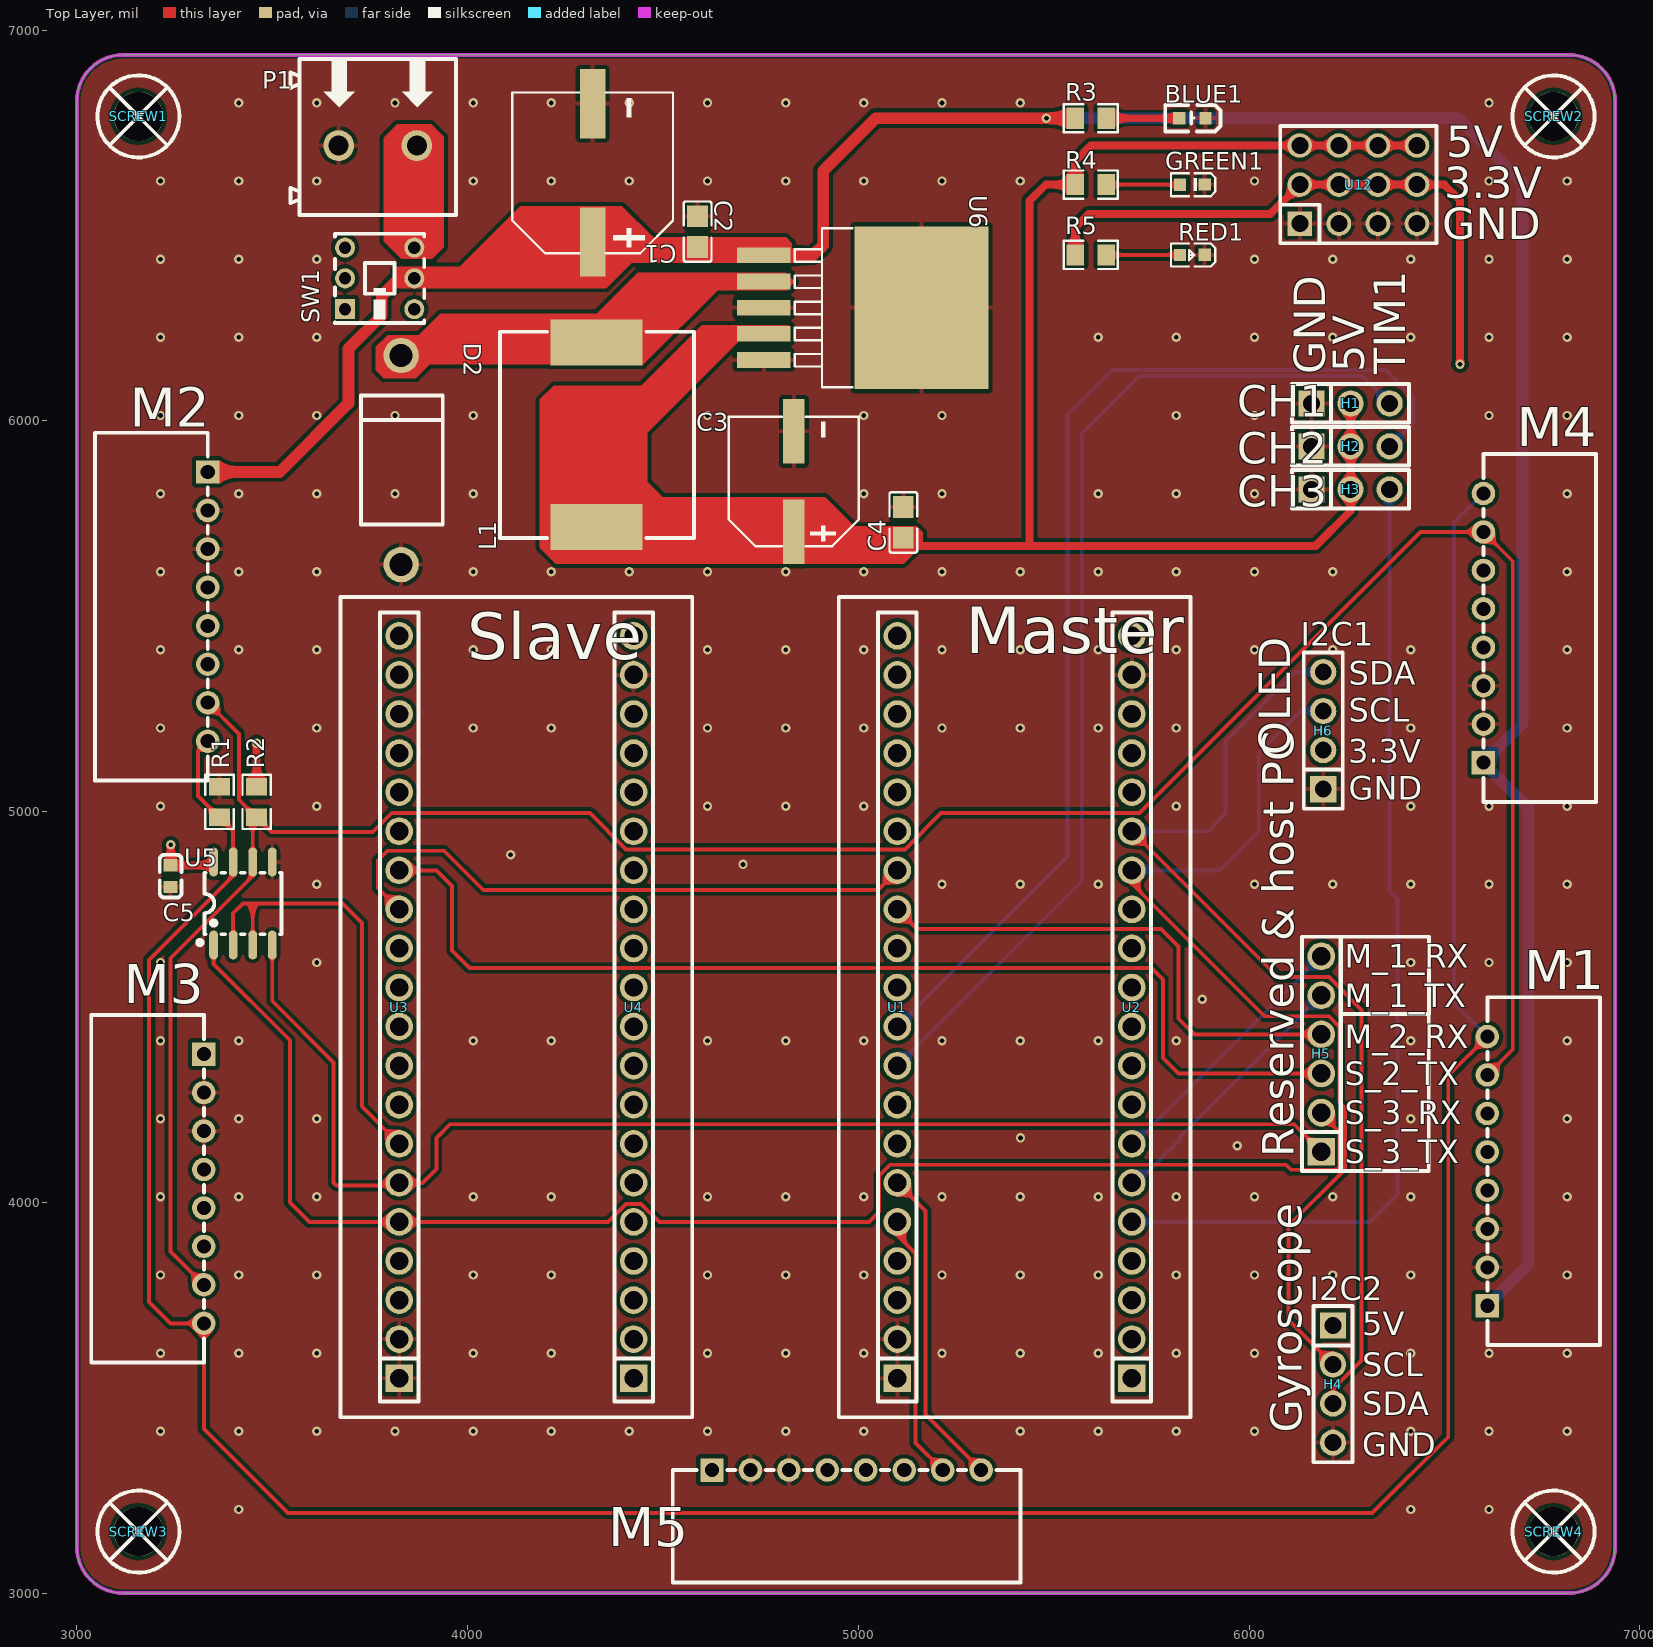
[diagram p0: Top Layer view]
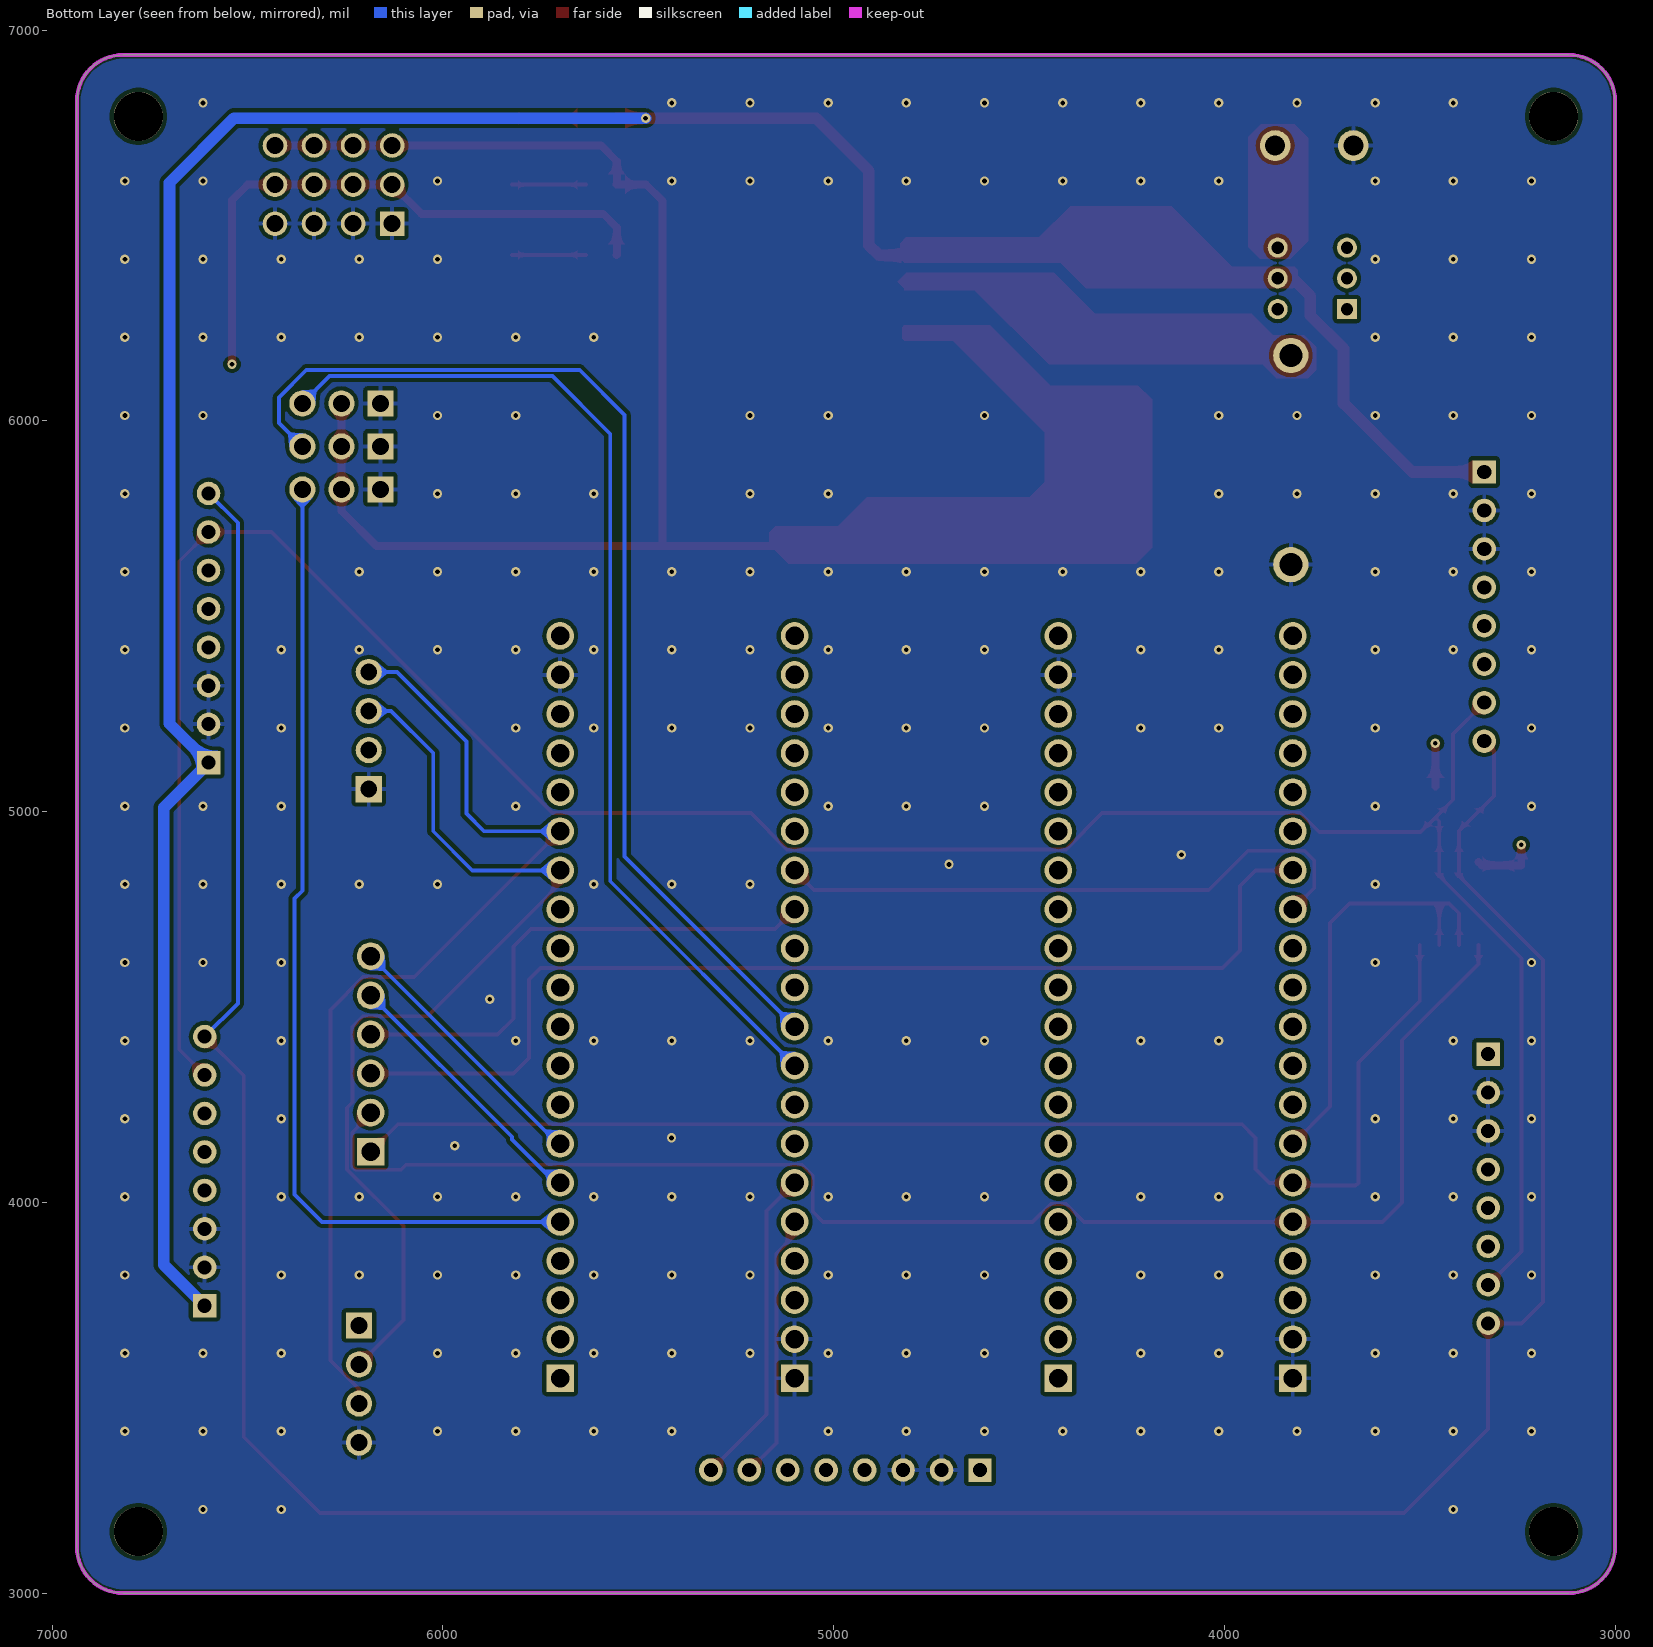
[diagram p1: Bottom Layer view, seen from below]
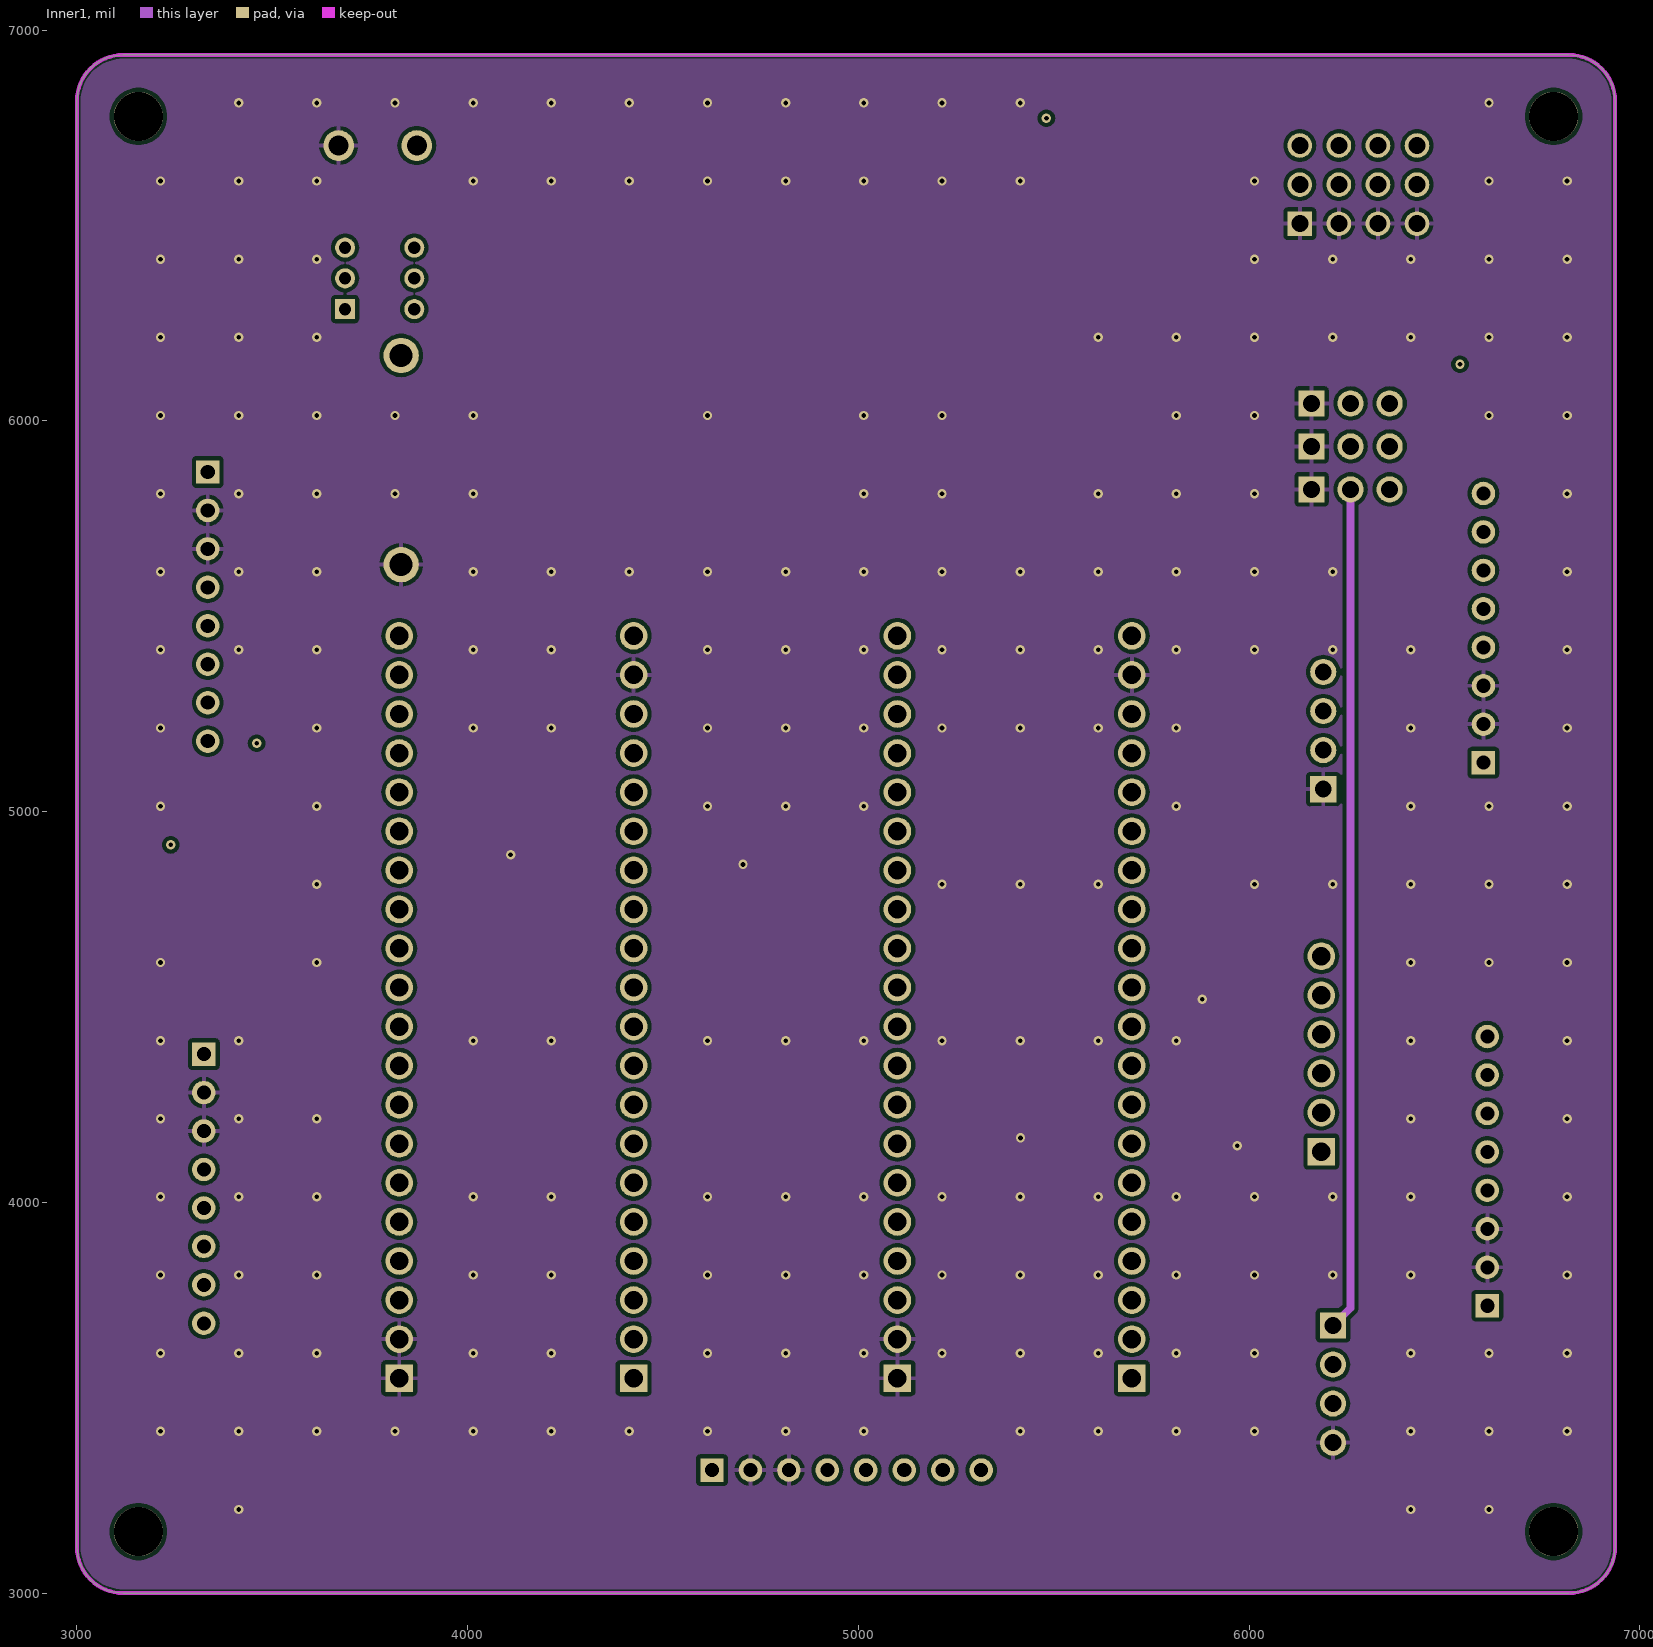
[diagram p2: Inner1]
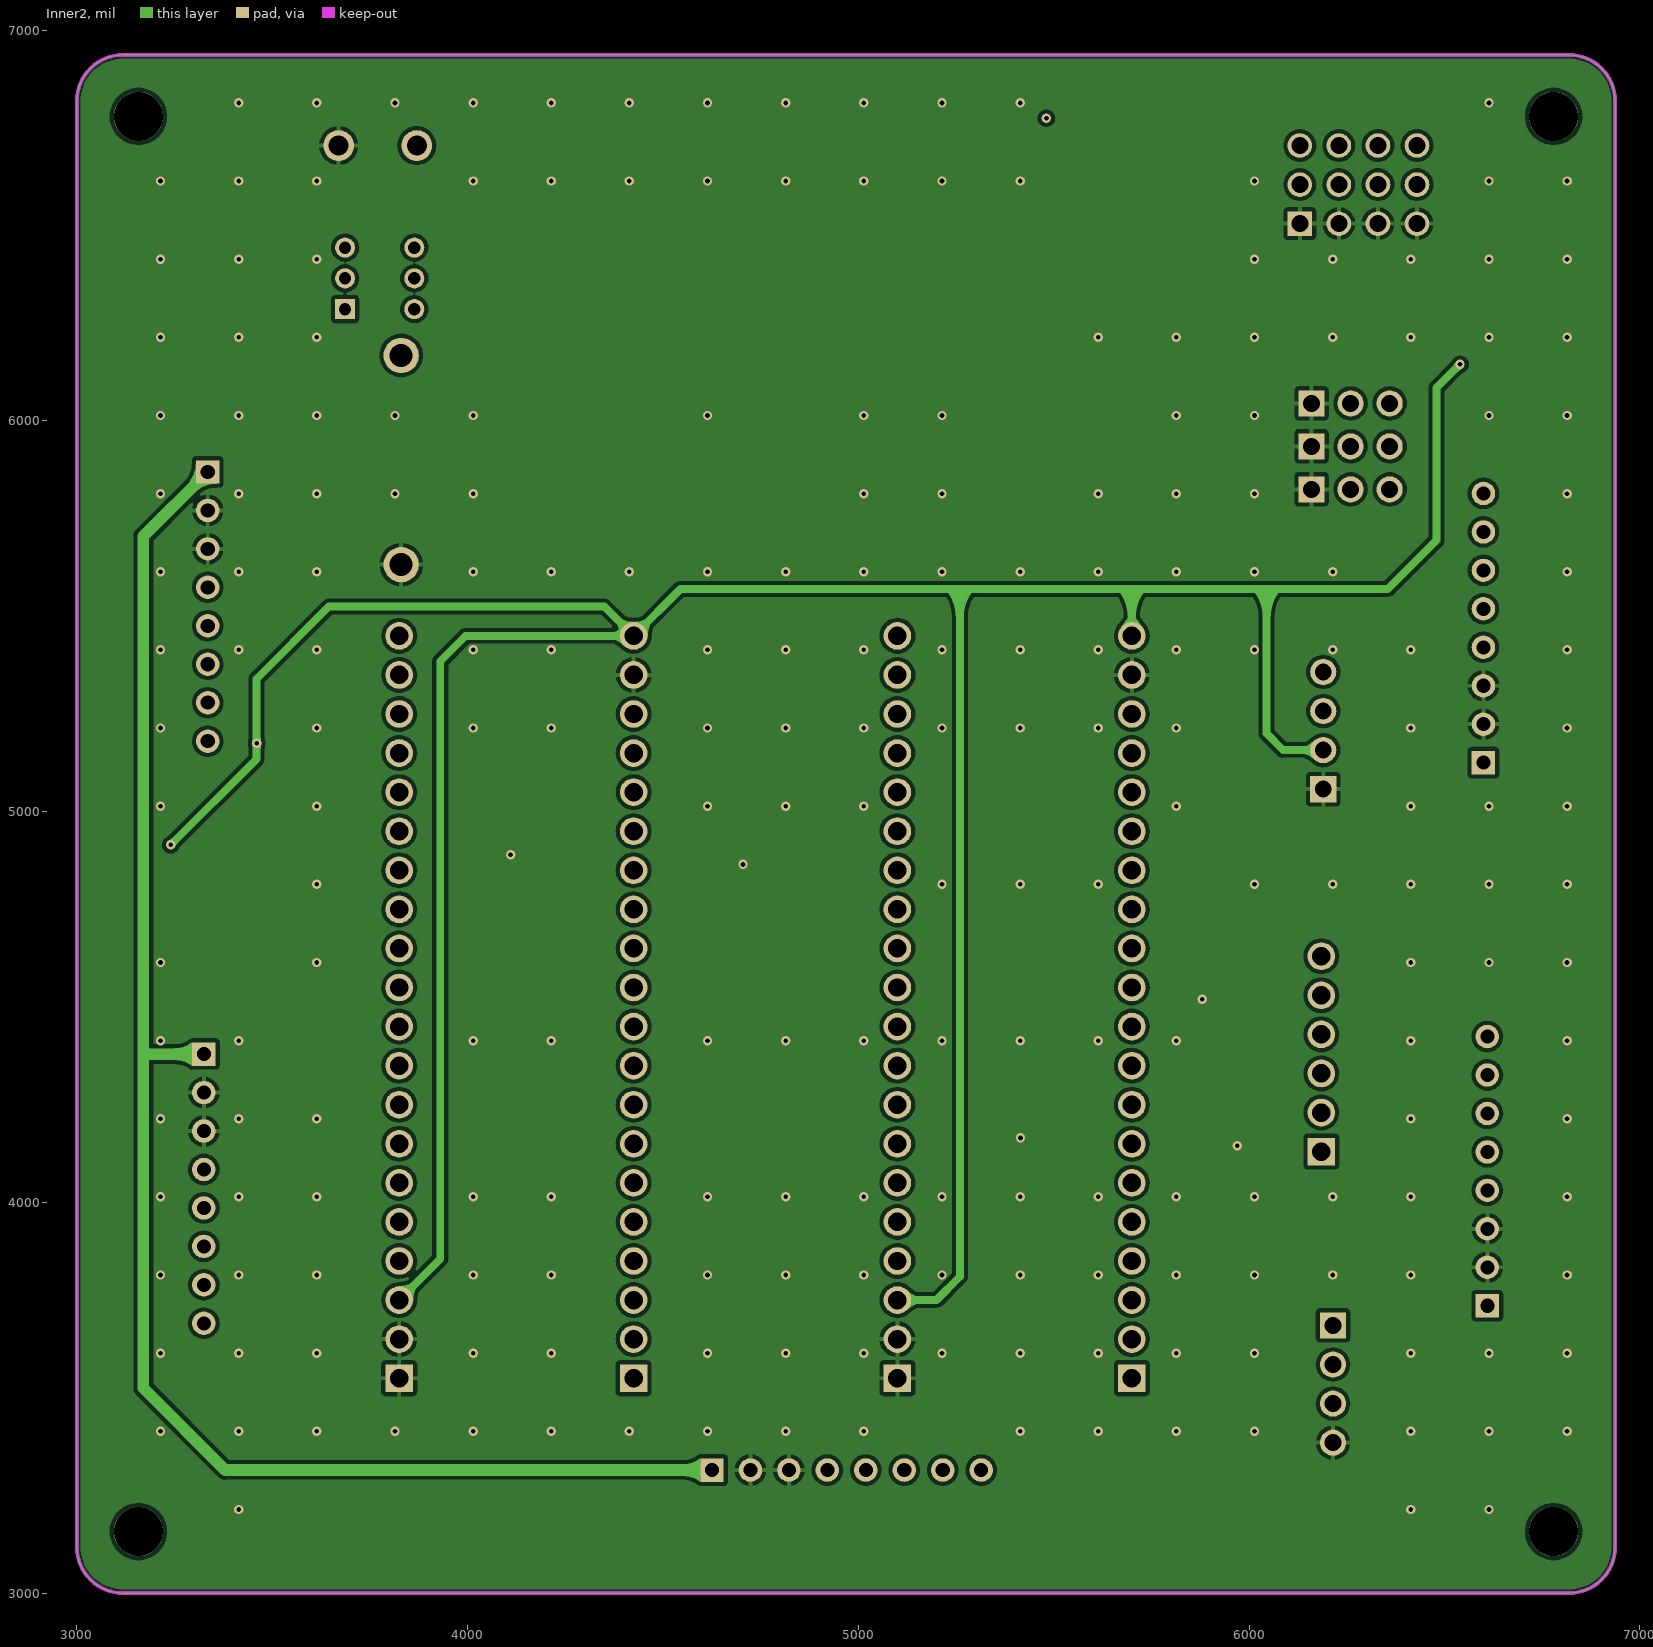
[diagram p3: Inner2]
# Altium PCB MISC50151.pcbdoc (part 1 of 4)
Units mil, origin at the board's own origin, x right, y up, seen from the top; angles counter-clockwise.
Board outline 3937.01 x 3937.01 mil, 4 copper layers (Top Layer, Inner1, Inner2, Bottom Layer), stack 62.447 mil thick; 39 components, 26 nets, 211 pads, 230 vias.

## Layer stack, top to bottom
Top Layer: signal copper 1.378
Dielectric1: surface 8.283, 7628 RC49% 8.6mil, Dk 0
Inner1: signal copper 0.598
Dielectric2: surface 41.929, 1.1mm H/HOZ Copper, Dk 0
Inner2: signal copper 0.598
Dielectric3: surface 8.283, 7628 RC49% 8.6mil, Dk 0
Bottom Layer: signal copper 1.378

## Board outline
3118.11,6937.01 ccw(c3118.11,6818.9) 3000,6818.9 3000,3118.11 ccw(c3118.11,3118.11) 3118.11,3000 6818.9,3000 ccw(c6818.9,3118.11) 6937.01,3118.11 6937.01,6818.9 ccw(c6818.9,6818.9) 6818.9,6937.01 3118.11,6937.01

## Design rules (kind name [scope] priority, off if disabled: settings)
BoardOutlineClearance copperThickness2oz_1 [All] p2 off: genericclearance=7.99 ignorepadtopadclearanceinfootprint=FALSE except(0: Arc-SplitContinuation Track-SplitContinuation SMDPad-SplitContinuation THPad-SplitContinuation Via-SplitContinuation Fill-SplitContinuation Region-SplitContinuation Poly-SplitContinuation Text-SplitContinuation Hole-SplitContinuation; 5.98: Arc-CutoutEdge Track-CutoutEdge SMDPad-CutoutEdge THPad-CutoutEdge Via-CutoutEdge Text-CutoutEdge; 6.9: Hole-OutlineEdge Hole-CutoutEdge; 10: Poly-OutlineEdge Poly-CutoutEdge; 11.81: Arc-OutlineEdge Track-OutlineEdge SMDPad-OutlineEdge THPad-OutlineEdge Via-OutlineEdge Fill-OutlineEdge Region-OutlineEdge Text-OutlineEdge Fill-CutoutEdge Region-CutoutEdge)
BoardOutlineClearance Plane_innerPlane_1 [All] p4 off: genericclearance=4.02 ignorepadtopadclearanceinfootprint=FALSE except(0: Arc-SplitContinuation Track-SplitContinuation SMDPad-SplitContinuation THPad-SplitContinuation Via-SplitContinuation Fill-SplitContinuation Region-SplitContinuation Poly-SplitContinuation Text-SplitContinuation Hole-SplitContinuation; 5.98: Arc-CutoutEdge Track-CutoutEdge SMDPad-CutoutEdge THPad-CutoutEdge Via-CutoutEdge Text-CutoutEdge; 6.9: Hole-OutlineEdge Hole-CutoutEdge; 10: Poly-OutlineEdge Poly-CutoutEdge; 11.81: Arc-OutlineEdge Track-OutlineEdge SMDPad-OutlineEdge THPad-OutlineEdge Via-OutlineEdge Fill-OutlineEdge Region-OutlineEdge Text-OutlineEdge Fill-CutoutEdge Region-CutoutEdge)
BoardOutlineClearance Copper_copperRegion_1 [All] p6 off: genericclearance=4.02 ignorepadtopadclearanceinfootprint=FALSE except(0: Arc-SplitContinuation Track-SplitContinuation SMDPad-SplitContinuation THPad-SplitContinuation Via-SplitContinuation Fill-SplitContinuation Region-SplitContinuation Poly-SplitContinuation Text-SplitContinuation Hole-SplitContinuation; 5.98: Arc-CutoutEdge Track-CutoutEdge SMDPad-CutoutEdge THPad-CutoutEdge Via-CutoutEdge Text-CutoutEdge; 6.9: Hole-OutlineEdge Hole-CutoutEdge; 10: Poly-OutlineEdge Poly-CutoutEdge; 11.81: Arc-OutlineEdge Track-OutlineEdge SMDPad-OutlineEdge THPad-OutlineEdge Via-OutlineEdge Fill-OutlineEdge Region-OutlineEdge Text-OutlineEdge Fill-CutoutEdge Region-CutoutEdge)
BoardOutlineClearance copperThickness1oz_1 [All] p8: genericclearance=4.02 ignorepadtopadclearanceinfootprint=FALSE except(0: Arc-SplitContinuation Track-SplitContinuation SMDPad-SplitContinuation THPad-SplitContinuation Via-SplitContinuation Fill-SplitContinuation Region-SplitContinuation Poly-SplitContinuation Text-SplitContinuation Hole-SplitContinuation; 5.98: Arc-CutoutEdge Track-CutoutEdge SMDPad-CutoutEdge THPad-CutoutEdge Via-CutoutEdge Text-CutoutEdge; 6.9: Hole-OutlineEdge Hole-CutoutEdge; 10: Poly-OutlineEdge Poly-CutoutEdge; 11.81: Arc-OutlineEdge Track-OutlineEdge SMDPad-OutlineEdge THPad-OutlineEdge Via-OutlineEdge Fill-OutlineEdge Region-OutlineEdge Text-OutlineEdge Fill-CutoutEdge Region-CutoutEdge)
Clearance copperThickness2oz [All] p1 off: gap=7.99 ignorepadtopadclearanceinfootprint=FALSE except(5.98: SMDPad-Track SMDPad-SMDPad THPad-Track SMDPad-THPad THPad-THPad Track-Via SMDPad-Via THPad-Via Via-Via Fill-SMDPad Region-SMDPad Fill-THPad Region-THPad Fill-Via Region-Via Fill-Fill Fill-Region Region-Region Arc-Track Arc-SMDPad Arc-THPad Arc-Via Fill-Arc Region-Arc Arc-Arc Text-Track SMDPad-Text Text-THPad Text-Via Fill-Text Region-Text Arc-Text Text-Text; 6.9: Hole-Track Hole-SMDPad Hole-THPad Hole-Via Fill-Hole Region-Hole Hole-Arc Hole-Text; 10: Poly-Track Poly-SMDPad Poly-THPad Poly-Via Poly-Fill Poly-Region Poly-Poly Poly-Arc Poly-Text Poly-Hole; 11.81: Fill-Track Region-Track)
Clearance Plane_innerPlane [All] p3 off: gap=4.02 ignorepadtopadclearanceinfootprint=FALSE except(5.98: SMDPad-Track SMDPad-SMDPad THPad-Track SMDPad-THPad THPad-THPad Track-Via SMDPad-Via THPad-Via Via-Via Fill-SMDPad Region-SMDPad Fill-THPad Region-THPad Fill-Via Region-Via Fill-Fill Fill-Region Region-Region Arc-Track Arc-SMDPad Arc-THPad Arc-Via Fill-Arc Region-Arc Arc-Arc Text-Track SMDPad-Text Text-THPad Text-Via Fill-Text Region-Text Arc-Text Text-Text; 6.9: Hole-Track Hole-SMDPad Hole-THPad Hole-Via Fill-Hole Region-Hole Hole-Arc Hole-Text; 10: Poly-Track Poly-SMDPad Poly-THPad Poly-Via Poly-Fill Poly-Region Poly-Poly Poly-Arc Poly-Text Poly-Hole; 11.81: Fill-Track Region-Track)
Clearance Copper_copperRegion [All] p5 off: gap=4.02 ignorepadtopadclearanceinfootprint=FALSE except(5.98: SMDPad-Track SMDPad-SMDPad THPad-Track SMDPad-THPad THPad-THPad Track-Via SMDPad-Via THPad-Via Via-Via Fill-SMDPad Region-SMDPad Fill-THPad Region-THPad Fill-Via Region-Via Fill-Fill Fill-Region Region-Region Arc-Track Arc-SMDPad Arc-THPad Arc-Via Fill-Arc Region-Arc Arc-Arc Text-Track SMDPad-Text Text-THPad Text-Via Fill-Text Region-Text Arc-Text Text-Text; 6.9: Hole-Track Hole-SMDPad Hole-THPad Hole-Via Fill-Hole Region-Hole Hole-Arc Hole-Text; 10: Poly-Track Poly-SMDPad Poly-THPad Poly-Via Poly-Fill Poly-Region Poly-Poly Poly-Arc Poly-Text Poly-Hole; 11.81: Fill-Track Region-Track)
Clearance copperThickness1oz [All] p7: gap=4.02 ignorepadtopadclearanceinfootprint=FALSE except(5.98: SMDPad-Track SMDPad-SMDPad THPad-Track SMDPad-THPad THPad-THPad Track-Via SMDPad-Via THPad-Via Via-Via Fill-SMDPad Region-SMDPad Fill-THPad Region-THPad Fill-Via Region-Via Fill-Fill Fill-Region Region-Region Arc-Track Arc-SMDPad Arc-THPad Arc-Via Fill-Arc Region-Arc Arc-Arc Text-Track SMDPad-Text Text-THPad Text-Via Fill-Text Region-Text Arc-Text Text-Text; 6.9: Hole-Track Hole-SMDPad Hole-THPad Hole-Via Fill-Hole Region-Hole Hole-Arc Hole-Text; 10: Poly-Track Poly-SMDPad Poly-THPad Poly-Via Poly-Fill Poly-Region Poly-Poly Poly-Arc Poly-Text Poly-Hole; 11.81: Fill-Track Region-Track)
DiffPairsRouting differentialPair [All] p1: maxlimit=6 minlimit=6 mostfreqgap=6 toplayer_minwidth=5 toplayer_prefwidth=10 toplayer_maxwidth=100 toplayer_mingap=6 toplayer_prefgap=6 toplayer_maxgap=6 midlayer1_minwidth=5 midlayer1_prefwidth=10 midlayer1_maxwidth=100 midlayer1_mingap=6 midlayer1_prefgap=6 midlayer1_maxgap=6 midlayer2_minwidth=5 midlayer2_prefwidth=10 midlayer2_maxwidth=100 midlayer2_mingap=6 midlayer2_prefgap=6 midlayer2_maxgap=6 bottomlayer_minwidth=5 bottomlayer_prefwidth=10 bottomlayer_maxwidth=100 bottomlayer_mingap=6 bottomlayer_prefgap=6 bottomlayer_maxgap=6 maxuncoupledlength=10
HoleToHoleClearance otherClearance [All] p1: gap=11.81 allowstackedmicrovias=TRUE
Length netLength [All] p1: minlimit=0 maxlimit=0
MatchedLengths netLengthTolerance [All] p1: tolerance=1000
PasteMaskExpansion pasteMaskExpansion [All] p1: expansion=0
PlaneConnect innerPlane [All] p1: planeconnectstyle=Relief reliefexpansion=20 reliefentries=4 reliefconductorwidth=10 reliefairgap=10
PolygonConnect copperRegion [All] p1: connectstyle=Relief reliefconductorwidth=10 reliefentries=4 polygonreliefangle="90 Angle" airgapwidth=10 via.connectstyle=Relief via.reliefconductorwidth=10 via.reliefentries=4 via.polygonreliefangle="90 Angle" via.airgapwidth=10
RoutingVias viaSize [All] p1: holewidth=12.01 width=24.02 viastyle="Through Hole" minholewidth=11.81 minwidth=19.68 maxholewidth=248.03 maxwidth=393.7
SolderMaskExpansion solderMaskExpansion [IsVia] p1: expansion=-1000 istentingtop=TRUE
SolderMaskExpansion solderMaskExpansion [All] p2: expansion=2 istentingtop=FALSE
Width copperThickness2oz_2 [All] p1 off: maxlimit=100 minlimit=8 preferedwidth=10
Width 20mil [(InNet('5V') OR InNet('3.3V'))] p2: maxlimit=100 minlimit=5 preferedwidth=20
Width 30mil [(InNet('12.6V'))] p3: maxlimit=100 minlimit=5 preferedwidth=30
Width copperThickness1oz_2 [All] p4: maxlimit=100 minlimit=5 preferedwidth=10

## Components (designator, comment, footprint, x,y, rotation, side; value= is the part's Value field where it differs from the comment)
BLUE1 "SZYY0603B" LED0603-R-RD_BLUE 5855,6775 r180 top
C1 "220uF" CAP-SMD_BD10.0-L10.3-W10.3-FD 4320,6635 r90 top
C2 "100nF" C0805 4588.54,6484.65 r270 top
C3 "680uF" CAP-SMD_BD8.0-L8.3-W8.3-FD 4835,5845 r90 top
C4 "100nF" C0805 5115.27,5740.28 r270 top
C5 "100nF" C0603 3240,4835 r270 top
D2 "1N5824" DO-27_BD5.3-L8.4-P12.40-D1.3-RD 3830,5900 r270 top
GREEN1 "XL-1608PGC-06" LED0603-RD_GREEN 5855,6605 r180 top
H1 "PZ254V-11-03P" HDR-TH_3P-P2.54-V-M 6260,6045 r0 top
H2 "PZ254V-11-03P" HDR-TH_3P-P2.54-V-M 6260,5935 r0 top
H3 "PZ254V-11-03P" HDR-TH_3P-P2.54-V-M 6260,5825 r0 top
H4 "PZ254V-11-04P" HDR-TH_4P-P2.54-V-M 6215,3535 r270 top
H5 "2.54-1x6P straight pin" HDR-TH_6P-P2.54-V-M-1 6185,4380 r90 top
H6 "PZ254V-11-04P" HDR-TH_4P-P2.54-V-M 6190,5207.57 r90 top
L1 "33uH" IND-SMD_L13.45-W12.6 4330,5965 r90 top
M1 "ZX-XH2.54-8PWZ" CONN-TH_8P-P2.50_ZX-XH2.54-8PWZ 6610,4080 r90 top
M2 "ZX-XH2.54-8PWZ" CONN-TH_8P-P2.50_ZX-XH2.54-8PWZ 3335,5525 r270 top
M3 "ZX-XH2.54-8PWZ" CONN-TH_8P-P2.50_ZX-XH2.54-8PWZ 3325,4035 r270 top
M4 "ZX-XH2.54-8PWZ" CONN-TH_8P-P2.50_ZX-XH2.54-8PWZ 6600,5470 r90 top
M5 "ZX-XH2.54-8PWZ" CONN-TH_8P-P2.50_ZX-XH2.54-8PWZ 4970,3315 r0 top
P1 "WJ500V-5.08-2P" CONN-TH_2P-P5.00_WJ500V-5.08-2P 3770,6705 r0 top
R1 "4.7kΩ" R0805 3365,5025 r90 top
R2 "4.7kΩ" R0805 3460,5025 r90 top
R3 "3K" R0805 5595,6775 r180 top
R4 "1K" R0805 5595,6605 r180 top
R5 "550Ω" R0805 5595,6425 r180 top
RED1 "XL-1608SURC-06" LED0603-RD_RED 5855,6425 r180 top
SCREW1 "" M3螺丝 3157.48,6779.53 r0 top
SCREW2 "" M3螺丝 6779.53,6779.53 r0 top
SCREW3 "" M3螺丝 3157.48,3157.48 r0 top
SCREW4 "" M3螺丝 6779.53,3157.48 r0 top
SW1 "5.8 WSPT" SW-TH_6P-L5.8-W5.8-P2.00-LS4.5-TL_K8-5851E-L1 3775,6365 r90 top
U1 "ZX-PM2.54-1-20PY" HDR-TH_20P-P2.54-V-F 5100,4500 r90 top
U2 "ZX-PM2.54-1-20PY" HDR-TH_20P-P2.54-V-F 5700,4500 r90 top
U3 "ZX-PM2.54-1-20PY" HDR-TH_20P-P2.54-V-F 3825,4500 r90 top
U4 "ZX-PM2.54-1-20PY" HDR-TH_20P-P2.54-V-F 4425,4500 r90 top
U5 "MAX3485ESA-MS" SO-8_L4.9-W3.9-P1.27-LS5.9-BL 3425,4765 r0 top
U6 "LM2596S-ADJ" TO-263-5_L10.2-W8.6-P1.70-LS14.4-BR 4960,6290 r180 top
U12 "HX PZ2.54-3x4P ZZ" HDR-TH_12P-P2.54-V-M-R3-C4-S2.54 6280,6605 r0 top

## Footprints (in the part's own frame and the unit in brackets; to place one, negate y for a bottom-side part, rotate by r counter-clockwise, add the part's x,y. Pads: shape width x height; smd on the part's side, far side on the other; paste and mask are expansions set on the pad)
C0603 [mm]
  rect 0.8x0.9 smd: 1(-0.7,0) 2(0.7,0)
  silkscreen extent -1.39,-0.71 1.39,0.71
C0805 [mm]
  rect 1.41x1.35 smd paste-100 mask+0.051: 1(-1,0) 2(1,0)
  silkscreen extent -1.96,-0.9 1.96,0.9
CAP-SMD_BD8.0-L8.3-W8.3-FD [mm]
  rect 4.2x1.4 smd paste+0 mask+0.051: 1(-3.267,0) 2(3.267,0)
  silkscreen extent -4.2,-4.23 4.2,4.23
CAP-SMD_BD10.0-L10.3-W10.3-FD [mm]
  rect 4.5x1.65 smd paste+0 mask+0.051: 1(-4.5,0) 2(4.5,0)
  silkscreen extent -5.23,-5.23 5.23,5.23
CONN-TH_2P-P5.00_WJ500V-5.08-2P [mm]
  round 2 hole 1.3: 1(-2.54,0) 2(2.54,0)
  silkscreen extent -5.68,-4.52 5.08,5.64
CONN-TH_8P-P2.50_ZX-XH2.54-8PWZ [mil]
  rect 60x60 hole 36: 1(-344.49,0)
  round 60 hole 36: 2(-246.07,0) 3(-147.64,0) 4(-49.22,0) 5(49.21,0) 6(147.64,0) 7(246.06,0) 8(344.48,0)
  silkscreen extent -445,-288 445,0
DO-27_BD5.3-L8.4-P12.40-D1.3-RD [mm]
  round 2.3 hole 1.5 paste+0 mask+0.05: 1(-6.8,0) 2(6.8,0)
  silkscreen extent -4.2,-2.6 4.2,2.7
HDR-TH_3P-P2.54-V-M [mm]
  rect 1.7x1.7 hole 1.1: 1(-2.54,0)
  round 1.7 hole 1.1: 2(0,0) 3(2.54,0)
  silkscreen extent -3.81,-1.25 3.81,1.25
HDR-TH_4P-P2.54-V-M [mm]
  rect 1.7x1.7 hole 1.1: 1(-3.81,0)
  round 1.7 hole 1.1: 2(-1.27,0) 3(1.27,0) 4(3.81,0)
  silkscreen extent -5.08,-1.27 5.08,1.27
HDR-TH_6P-P2.54-V-M-1 [mm]
  rect 1.8x1.8 hole 1.2: 1(-6.35,0)
  round 1.8 hole 1.2: 2(-3.81,0) 3(-1.27,0) 4(1.27,0) 5(3.81,0) 6(6.35,0)
  silkscreen extent -7.62,-1.25 7.62,1.25
HDR-TH_12P-P2.54-V-M-R3-C4-S2.54 [mm]
  rect 1.6x1.6 hole 1.1 paste+0 mask+0.05: 1(-3.81,-2.54)
  round 1.6 hole 1.1 paste+0 mask+0.05: 2(-3.81,0) 3(-3.81,2.54) 4(-1.27,-2.54) 5(-1.27,0) 6(-1.27,2.54) 7(1.27,-2.54) 8(1.27,0) 9(1.27,2.54) 10(3.81,-2.54) 11(3.81,0) 12(3.81,2.54)
  silkscreen extent -5.08,-3.81 5.08,3.81
HDR-TH_20P-P2.54-V-F [mm]
  rect 1.8x1.8 hole 1.2: 1(-24.13,0)
  round 1.8 hole 1.2: 2(-21.59,0) 3(-19.05,0) 4(-16.51,0) 5(-13.97,0) 6(-11.43,0) 7(-8.89,0) 8(-6.35,0) 9(-3.81,0) 10(-1.27,0) 11(1.27,0) 12(3.81,0) 13(6.35,0) 14(8.89,0) 15(11.43,0) 16(13.97,0) 17(16.51,0) 18(19.05,0) 19(21.59,0) 20(24.13,0)
  silkscreen extent -25.65,-1.25 25.65,1.25
IND-SMD_L13.45-W12.6 [mm]
  rect 3x6 smd paste+0 mask+0.051: 1(-6,0) 2(6,0)
  silkscreen extent -6.71,-6.33 6.69,6.28
LED0603-R-RD_BLUE [mm]
  rect 0.8x0.8 smd: 1(0.851,0) 2(-0.851,0)
  silkscreen extent -1.82,-0.86 1.77,0.86
LED0603-RD_GREEN [mm]
  rect 0.8x0.8 smd: 1(-0.799,-0.003) 2(0.799,0.003)
  silkscreen extent -1.49,-0.75 1.39,0.76
LED0603-RD_RED [mm]
  rect 0.8x0.8 smd: 1(-0.8,-0.003) 2(0.8,0.003)
  silkscreen extent -1.49,-0.75 1.39,0.76
M3螺丝 [mil]
  round 126 hole 126 paste+0 mask+4: 1(0,0)
  silkscreen extent -105,-105 105,105
R0805 [mm]
  rect 1.133x1.377 smd paste-100 mask+0.051: 1(-1,0) 2(1,0)
  silkscreen extent -1.76,-0.92 1.76,0.92
SO-8_L4.9-W3.9-P1.27-LS5.9-BL [mil]
  oval 22.6x74.33 smd: 1(-75,-106.26) 2(-25,-106.26) 3(25,-106.26) 4(75,-106.26) 5(75,106.26) 6(25,106.26) 7(-25,106.26) 8(-75,106.26)
  silkscreen extent -116,-106 98,79
SW-TH_6P-L5.8-W5.8-P2.00-LS4.5-TL_K8-5851E-L1 [mm]
  rect 1.3x1.3 hole 0.8 paste+0 mask+0.05: 1(-2,2.25)
  round 1.3 hole 0.8 paste+0 mask+0.05: 2(0,2.25) 3(2,2.25) 4(-2,-2.25) 5(0,-2.25) 6(2,-2.25)
  silkscreen extent -2.9,-2.9 2.9,2.92
TO-263-5_L10.2-W8.6-P1.70-LS14.4-BR [mm]
  rect 3.5x1.02 smd paste+0 mask+0.051: 1(5.126,-3.4) 2(5.126,-1.7) 3(5.126,0) 4(5.126,1.7) 5(5.126,3.4)
  rect 8.705x10.587 smd paste+0 mask+0.051: 6(-5.126,0)
  silkscreen extent -0.62,-5.17 3.11,5.17

## Via types
v1: diameter 24.02, hole 12, Top Layer to Bottom Layer, 230 vias

## Nets (pads, with @x,y where several pads share a name; then routed paths per layer and width w, separated by ;. In a path a pad name is that pad's centre, name@x,y a point inside that pad or via, vN(x,y) a via of type N, cw(c..) or ccw(c..) an arc to the next point about the centre after c; other vN are vias at no path point)
3.3V: C5.1 H6.2 R2.2 R5.2 U1.3 U2.20 U3.3 U4.20 U5.8 U12.2 U12.5 U12.8 U12.11 | length 10834.1
  Top Layer w20: v1(3240,4915) C5.1@3240,4862.56 3341.3,4862.56 U5.8@3350,4871.26 ; R2.2@3460,5064.37 v1(3460,5175) ; R5.2@5555.63,6425 5555,6425.63 5555,6495 5590,6530 6055,6530 U12.2@6130,6605 U12.5@6230,6605 U12.8@6330,6605 U12.11@6430,6605 6500,6605 6540,6565 v1(6540,6145)
  Inner2 w20: v1(3240,4915) 3460,5135 v1(3460,5175) 3460,5340 3645,5525 4350,5525 U4.20@4425,5450 ; U3.3@3825,3750 3930,3855 3930,5385 3995,5450 U4.20@4425,5450 ; U1.3@5100,3750 5200,3750 5260,3810 5260,5570 ; U2.20@5700,5450 5700,5565 ; H6.2@6190,5157.57 6087.43,5157.57 6045,5200 6045,5570 ; v1(6540,6145) 6480,6085 6480,5695 6355,5570 6045,5570 ; U4.20@4425,5450 4545,5570 5260,5570 ; 5260,5570 5695,5570 5700,5565 ; 5700,5565 5700,5570 6045,5570
5V: C3.1 C4.2 H1.2 H2.2 H3.2 H4.1 L1.1 R4.2 U6.4 U12.3 U12.6 U12.9 U12.12 | length 5655.7
  Top Layer w20: 5045,5680 5438.27,5680 ; H1.2@6260,6045 H2.2@6260,5935 H3.2@6260,5825 6260,5770 6170,5680 5438.27,5680 ; U12.12@6430,6705 U12.9@6330,6705 U12.6@6230,6705 U12.3@6130,6705 5595,6705 5555,6665 5555,6605.63 R4.2@5555.63,6605 5480,6605 5438.27,6563.27 5438.27,5680
  Inner1 w20: H4.1@6215,3685 6260,3730 H3.2@6260,5825
12.6V: C1.1 C2.2 M1.1 M2.1 M3.1 M4.1 M5.1 R3.2 SW1.5 U6.1 | length 10304.9
  Top Layer w30: M2.1@3335,5869.49 3519.49,5869.49 3695,6045 3695,6185 3780,6270 3780,6320 3825,6365 SW1.5@3863.58,6365 ; U6.1@4758.17,6423.86 4883.86,6423.86 4910,6450 4910,6640 5045,6775 v1(5481.49,6775) R3.2@5555.63,6775
  Inner2 w30: M3.1@3325,4379.49 3173.19,4379.49 3170,4382.68 ; M2.1@3335,5869.49 3170,5704.49 3170,4382.68 ; M5.1@4625.51,3315 3380,3315 3170,3525 3170,4382.68
  Bottom Layer w30: v1(5481.49,6775) 6535,6775 6700,6610 6700,5225.51 M4.1@6600,5125.51 6715,5010.51 6715,3840.51 M1.1@6610,3735.51
$1N570: D2.1 L1.2 U6.2
$1N591: BLUE1.1 R3.1 | length 187.1
  Top Layer w20: R3.1@5634.37,6775 BLUE1.1@5821.5,6775
$1N595: GREEN1.2 R4.1 | length 189.2
  Top Layer w10: R4.1@5634.37,6605 5634.51,6604.86 GREEN1.2@5823.52,6604.86
$1N596: P1.2 SW1.6
$1N953: R5.1 RED1.2 | length 189.2
  Top Layer w10: R5.1@5634.37,6425 5823.39,6425 RED1.2@5823.52,6424.86
BUS_S_A: M1.7 M2.7 M3.7 M4.7 R2.1 U5.6 | length 6666.8
  Top Layer w10: M3.7@3325,3788.94 3240,3873.94 3240,4625 3450,4835 U5.6@3450,4871.26 3450,4975.63 R2.1@3460,4985.63 ; M2.7@3335,5278.94 3415,5198.94 3415,5030.63 R2.1@3460,4985.63 ; M1.7@6610,4326.06 6675,4391.06 6675,5641.06 M4.7@6600,5716.06 6438.87,5716.06 5719.23,4996.42 5212.06,4996.42 5119.23,4903.58 4405.77,4903.58 4312.94,4996.42 3805.77,4996.42 3757.32,4947.96 3497.67,4947.96 R2.1@3460,4985.63
BUS_S_B: M1.8 M2.8 M3.8 M4.8 R1.1 U5.7 | length 7882.3
  Top Layer w10: M2.8@3335,5180.52 3310,5155.51 3310,5040.63 R1.1@3365,4985.63 3400,4950.63 U5.7@3400,4871.26 3400,4835 3185,4620 3185,3745 3239.49,3690.51 M3.8@3325,3690.51 3325,3420 3540,3205 6315,3205 6510,3400 6510,4324.49 M1.8@6610,4424.48
  Bottom Layer w10: M4.8@6600,5814.48 6525,5739.49 6525,4509.49 M1.8@6610,4424.48